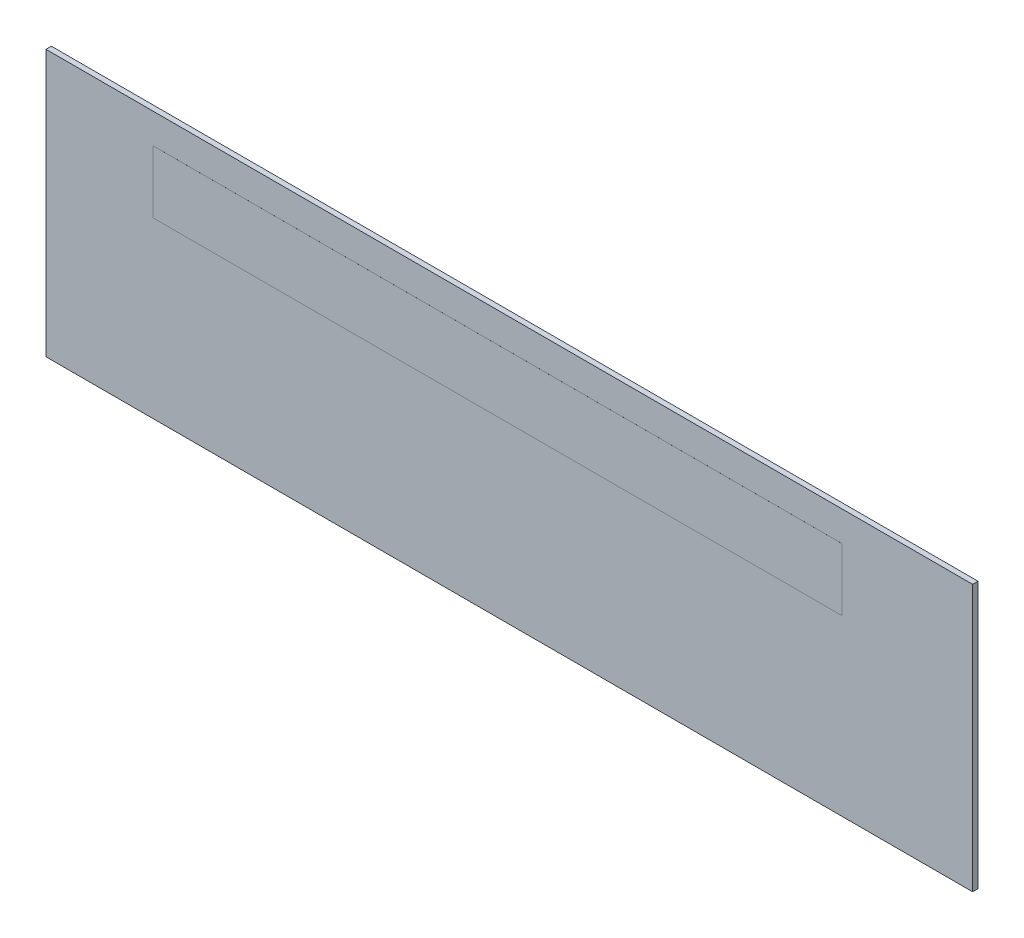
SolidWorks part; units mm, degrees
ref_plane "Frontal" through (0, 0, 0) normal (0, 0, 1) x (1, 0, 0)
ref_plane "Superior" through (0, 0, 0) normal (0, 1, 0) x (1, 0, 0)
ref_plane "Direito" through (0, 0, 0) normal (1, 0, 0) x (0, 0, -1)
sketch "Sketch1" plane through (0, 0, 0) normal (0, 0, 1) x (1, 0, 0)
  line L1 (-257.5, 74) -> (257.5, 74)
  line L2 (-257.5, 74) -> (-257.5, -74)
  line L3 (-257.5, -74) -> (257.5, -74)
  line L4 (257.5, 74) -> (257.5, -74)
  line L5 (-257.5, 74) -> (257.5, -74) construction
  line L6 (-257.5, -74) -> (257.5, 74) construction
  point P0 (0, 0)
  dimension "D1" = 148
  dimension "D2" = 515
extrude "Boss-Extrude1" add sketch "Sketch1" along normal blind 3
sketch "Sketch2" plane through (0, 0, 3) normal (0, 0, 1) x (1, 0, 0)
  line L3 (184.8563, 57.3277) -> (-198.1111, 57.3277)
  line L4 (184.8563, 57.3277) -> (184.8563, 22.6315)
  line L5 (184.8563, 22.6315) -> (-198.1111, 22.6315)
  line L6 (-198.1111, 57.3277) -> (-198.1111, 22.6315)
extrude "Boss-Extrude2" add sketch "Sketch2" along normal blind 0.01
